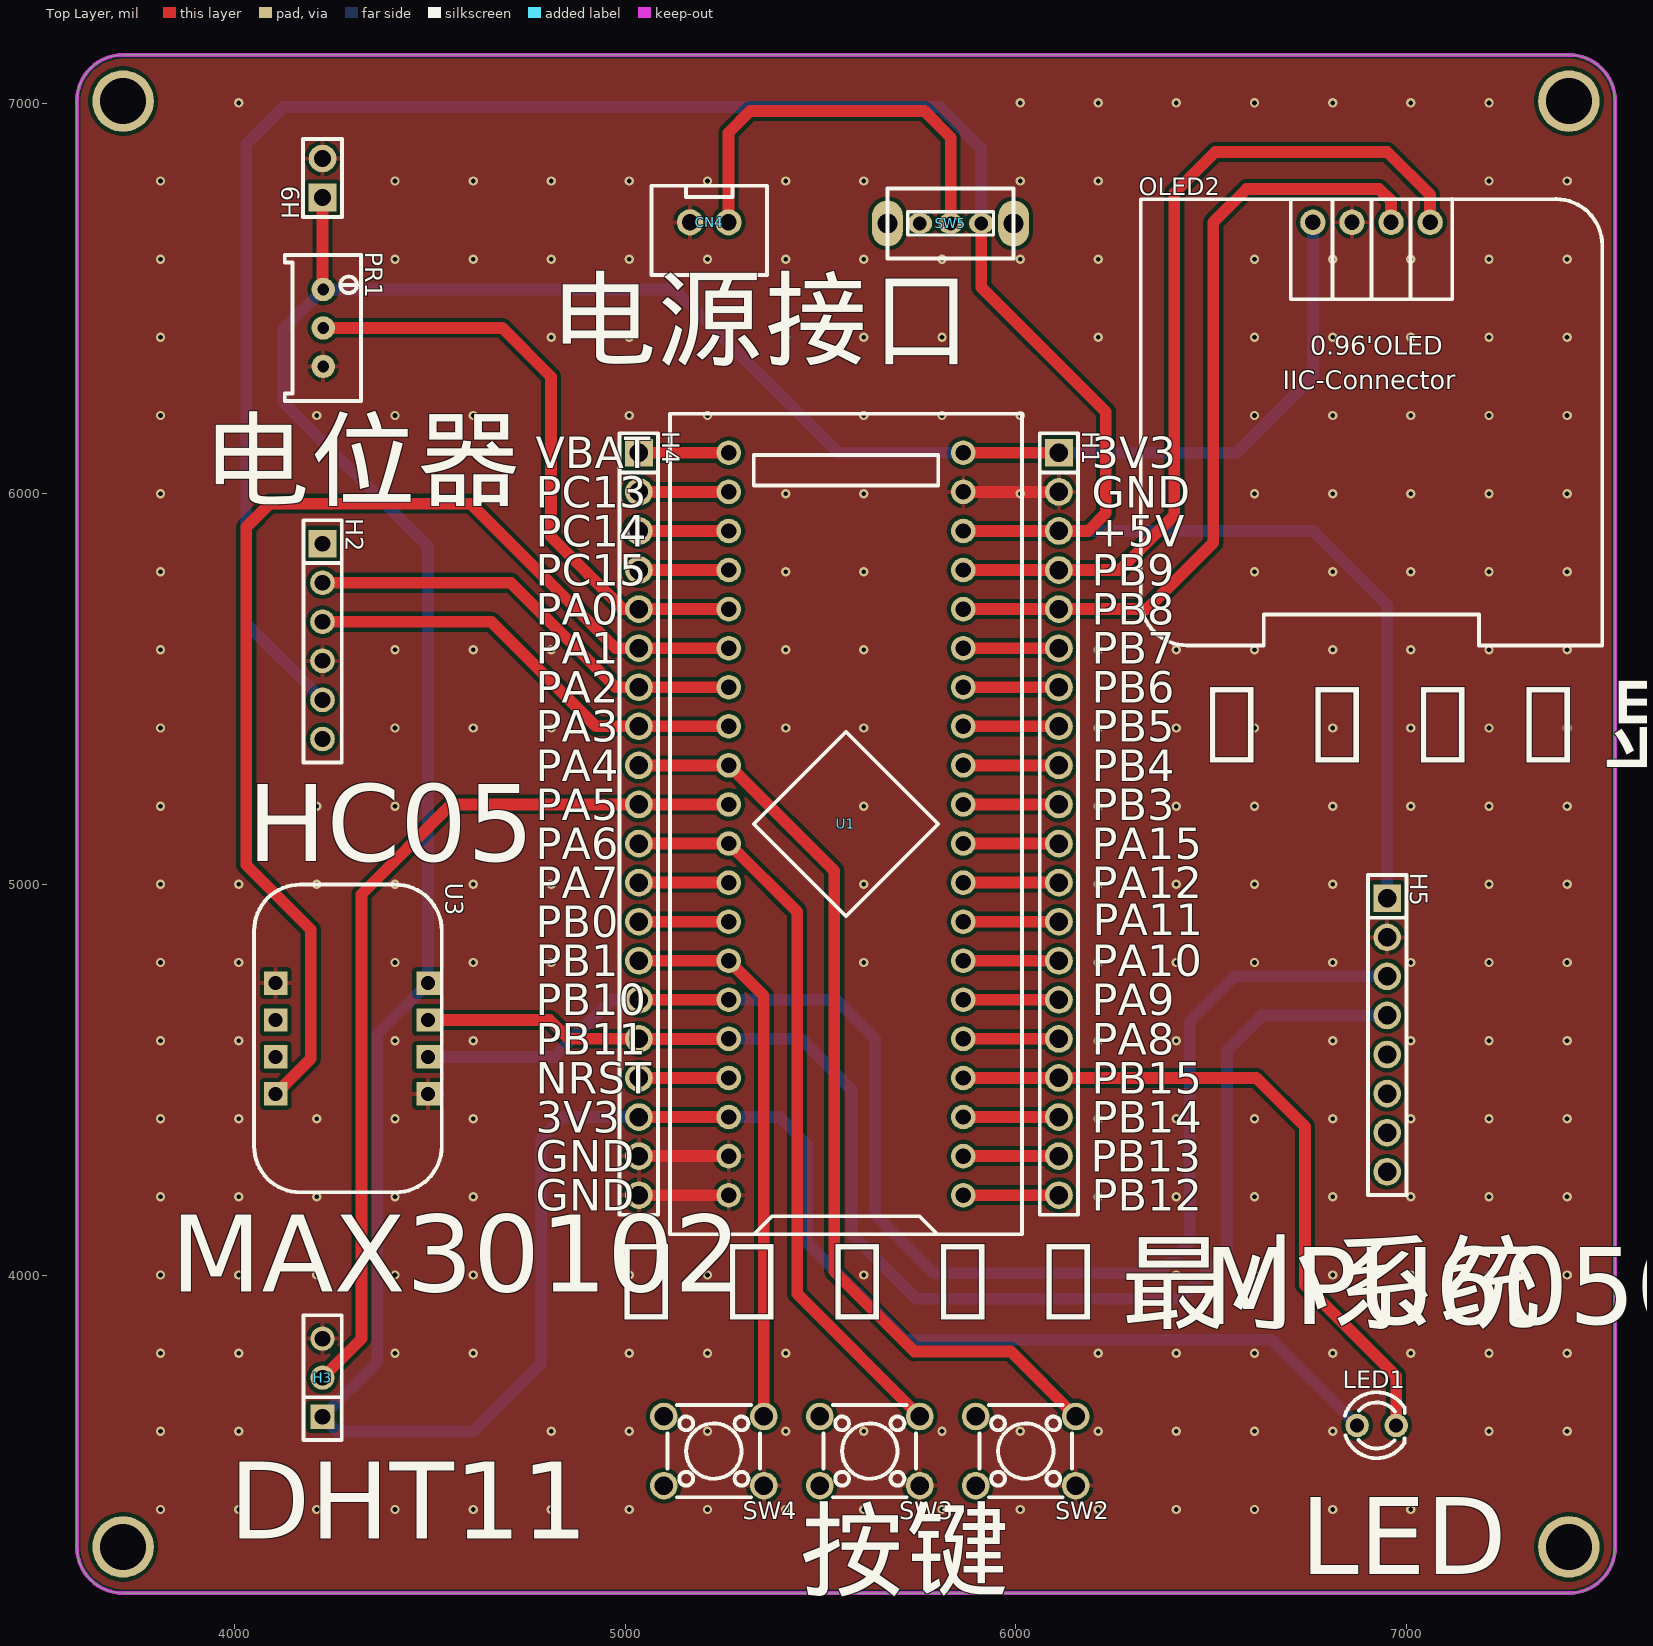
[diagram p0: Top Layer view]
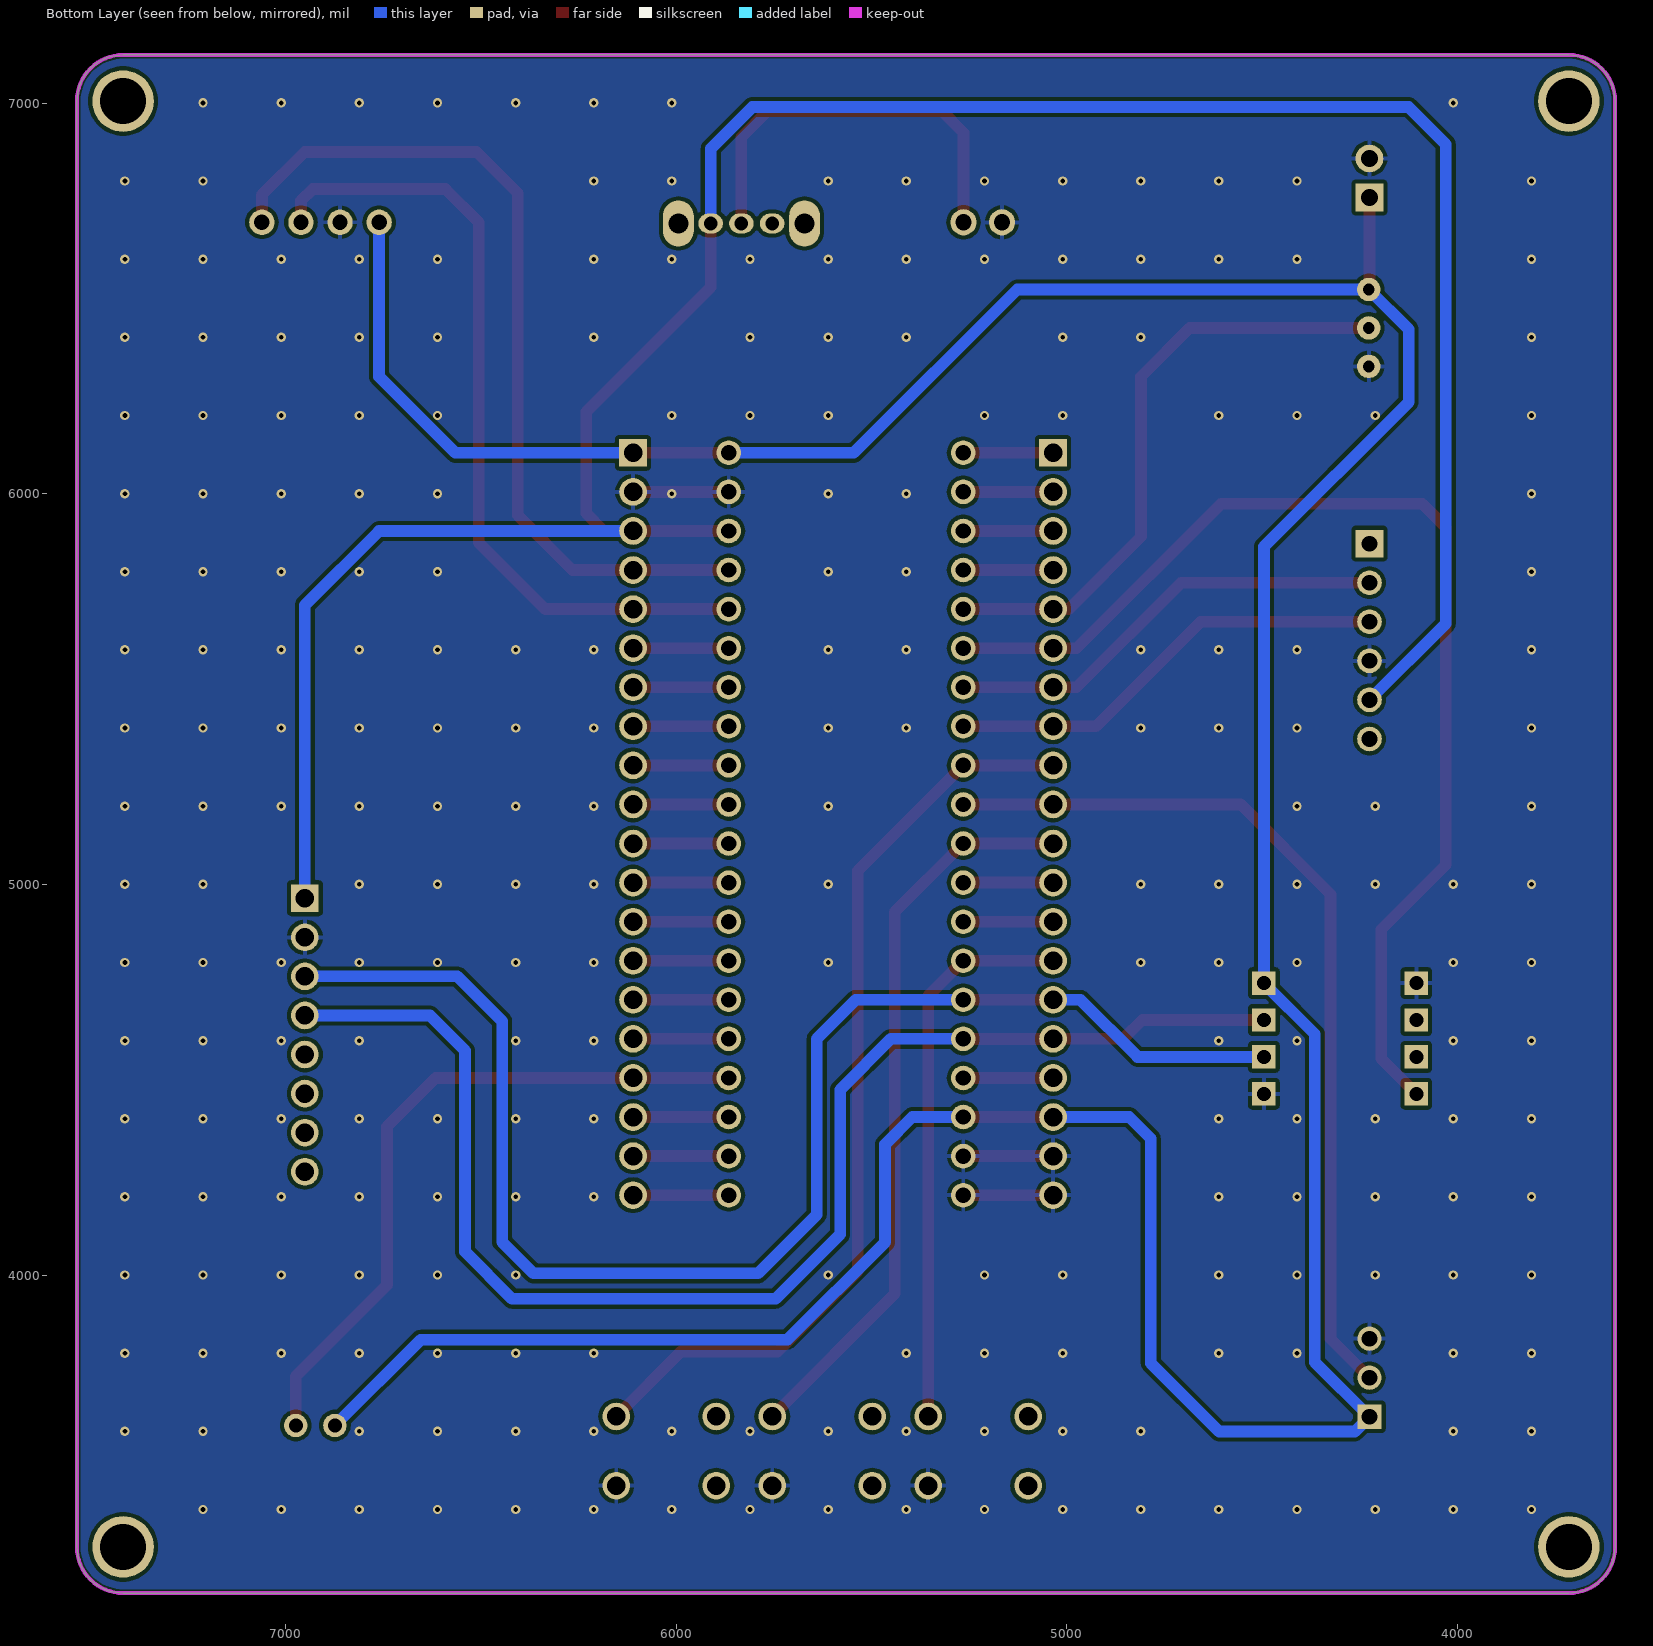
[diagram p1: Bottom Layer view, seen from below]
# Altium PCB MISC51261.pcbdoc
Units mil, origin at the board's own origin, x right, y up, seen from the top; angles counter-clockwise.
Board outline 3937.01 x 3937.01 mil, 2 copper layers (Top Layer, Bottom Layer), stack 62.206 mil thick; 16 components, 38 nets, 139 pads, 237 vias.

## Layer stack, top to bottom
Top Solder Mask Layer: solder mask 0.394, Dk 3.3
Top Layer: signal copper 1.379
Dielectric1: surface 59.449, FR4, Dk 4.5
Bottom Layer: signal copper 1.378
Bottom Solder Mask Layer: solder mask 0.394, Dk 3.3

## Board outline
3714.61,7123.5 ccw(c3714.61,7005.39) 3596.5,7005.39 3596.5,3304.61 ccw(c3714.61,3304.61) 3714.61,3186.5 7415.39,3186.5 ccw(c7415.39,3304.61) 7533.5,3304.61 7533.5,7005.39 ccw(c7415.39,7005.39) 7415.39,7123.5 3714.61,7123.5

## Design rules (kind name [scope] priority, off if disabled: settings)
BoardOutlineClearance copperThickness2oz_1 [All] p2 off: genericclearance=7.99 ignorepadtopadclearanceinfootprint=FALSE except(0: Arc-SplitContinuation Track-SplitContinuation SMDPad-SplitContinuation THPad-SplitContinuation Via-SplitContinuation Fill-SplitContinuation Region-SplitContinuation Poly-SplitContinuation Text-SplitContinuation Hole-SplitContinuation; 5.98: Arc-CutoutEdge Track-CutoutEdge SMDPad-CutoutEdge THPad-CutoutEdge Via-CutoutEdge Text-CutoutEdge; 6.9: Hole-OutlineEdge Hole-CutoutEdge; 10: Poly-OutlineEdge Poly-CutoutEdge; 11.81: Arc-OutlineEdge Track-OutlineEdge SMDPad-OutlineEdge THPad-OutlineEdge Via-OutlineEdge Fill-OutlineEdge Region-OutlineEdge Text-OutlineEdge Fill-CutoutEdge Region-CutoutEdge)
BoardOutlineClearance Plane_innerPlane_1 [All] p4 off: genericclearance=4.02 ignorepadtopadclearanceinfootprint=FALSE except(0: Arc-SplitContinuation Track-SplitContinuation SMDPad-SplitContinuation THPad-SplitContinuation Via-SplitContinuation Fill-SplitContinuation Region-SplitContinuation Poly-SplitContinuation Text-SplitContinuation Hole-SplitContinuation; 5.98: Arc-CutoutEdge Track-CutoutEdge SMDPad-CutoutEdge THPad-CutoutEdge Via-CutoutEdge Text-CutoutEdge; 6.9: Hole-OutlineEdge Hole-CutoutEdge; 10: Poly-OutlineEdge Poly-CutoutEdge; 11.81: Arc-OutlineEdge Track-OutlineEdge SMDPad-OutlineEdge THPad-OutlineEdge Via-OutlineEdge Fill-OutlineEdge Region-OutlineEdge Text-OutlineEdge Fill-CutoutEdge Region-CutoutEdge)
BoardOutlineClearance Copper_copperRegion_1 [All] p6 off: genericclearance=4.02 ignorepadtopadclearanceinfootprint=FALSE except(0: Arc-SplitContinuation Track-SplitContinuation SMDPad-SplitContinuation THPad-SplitContinuation Via-SplitContinuation Fill-SplitContinuation Region-SplitContinuation Poly-SplitContinuation Text-SplitContinuation Hole-SplitContinuation; 5.98: Arc-CutoutEdge Track-CutoutEdge SMDPad-CutoutEdge THPad-CutoutEdge Via-CutoutEdge Text-CutoutEdge; 6.9: Hole-OutlineEdge Hole-CutoutEdge; 10: Poly-OutlineEdge Poly-CutoutEdge; 11.81: Arc-OutlineEdge Track-OutlineEdge SMDPad-OutlineEdge THPad-OutlineEdge Via-OutlineEdge Fill-OutlineEdge Region-OutlineEdge Text-OutlineEdge Fill-CutoutEdge Region-CutoutEdge)
BoardOutlineClearance Copper_copperRegion_copperThickness1oz_1 [All] p8 off: genericclearance=4.02 ignorepadtopadclearanceinfootprint=FALSE except(0: Arc-SplitContinuation Track-SplitContinuation SMDPad-SplitContinuation THPad-SplitContinuation Via-SplitContinuation Fill-SplitContinuation Region-SplitContinuation Poly-SplitContinuation Text-SplitContinuation Hole-SplitContinuation; 5.98: Arc-CutoutEdge Track-CutoutEdge SMDPad-CutoutEdge THPad-CutoutEdge Via-CutoutEdge Text-CutoutEdge; 6.9: Hole-OutlineEdge Hole-CutoutEdge; 10: Poly-OutlineEdge Poly-CutoutEdge; 11.81: Arc-OutlineEdge Track-OutlineEdge SMDPad-OutlineEdge THPad-OutlineEdge Via-OutlineEdge Fill-OutlineEdge Region-OutlineEdge Text-OutlineEdge Fill-CutoutEdge Region-CutoutEdge)
BoardOutlineClearance Copper_copperRegion_Copper_copperRegion_1 [All] p10 off: genericclearance=4.02 ignorepadtopadclearanceinfootprint=FALSE except(0: Arc-SplitContinuation Track-SplitContinuation SMDPad-SplitContinuation THPad-SplitContinuation Via-SplitContinuation Fill-SplitContinuation Region-SplitContinuation Poly-SplitContinuation Text-SplitContinuation Hole-SplitContinuation; 5.98: Arc-CutoutEdge Track-CutoutEdge SMDPad-CutoutEdge THPad-CutoutEdge Via-CutoutEdge Text-CutoutEdge; 6.9: Hole-OutlineEdge Hole-CutoutEdge; 10: Poly-OutlineEdge Poly-CutoutEdge; 11.81: Arc-OutlineEdge Track-OutlineEdge SMDPad-OutlineEdge THPad-OutlineEdge Via-OutlineEdge Fill-OutlineEdge Region-OutlineEdge Text-OutlineEdge Fill-CutoutEdge Region-CutoutEdge)
BoardOutlineClearance copperThickness1oz_1 [All] p12: genericclearance=4.02 ignorepadtopadclearanceinfootprint=FALSE except(0: Arc-SplitContinuation Track-SplitContinuation SMDPad-SplitContinuation THPad-SplitContinuation Via-SplitContinuation Fill-SplitContinuation Region-SplitContinuation Poly-SplitContinuation Text-SplitContinuation Hole-SplitContinuation; 5.98: Arc-CutoutEdge Track-CutoutEdge SMDPad-CutoutEdge THPad-CutoutEdge Via-CutoutEdge Text-CutoutEdge; 6.9: Hole-OutlineEdge Hole-CutoutEdge; 10: Poly-OutlineEdge Poly-CutoutEdge; 11.81: Arc-OutlineEdge Track-OutlineEdge SMDPad-OutlineEdge THPad-OutlineEdge Via-OutlineEdge Fill-OutlineEdge Region-OutlineEdge Text-OutlineEdge Fill-CutoutEdge Region-CutoutEdge)
Clearance copperThickness2oz [All] p1 off: gap=7.99 ignorepadtopadclearanceinfootprint=FALSE except(5.98: SMDPad-Track SMDPad-SMDPad THPad-Track SMDPad-THPad THPad-THPad Track-Via SMDPad-Via THPad-Via Via-Via Fill-SMDPad Region-SMDPad Fill-THPad Region-THPad Fill-Via Region-Via Fill-Fill Fill-Region Region-Region Arc-Track Arc-SMDPad Arc-THPad Arc-Via Fill-Arc Region-Arc Arc-Arc Text-Track SMDPad-Text Text-THPad Text-Via Fill-Text Region-Text Arc-Text Text-Text; 6.9: Hole-Track Hole-SMDPad Hole-THPad Hole-Via Fill-Hole Region-Hole Hole-Arc Hole-Text; 10: Poly-Track Poly-SMDPad Poly-THPad Poly-Via Poly-Fill Poly-Region Poly-Poly Poly-Arc Poly-Text Poly-Hole; 11.81: Fill-Track Region-Track)
Clearance Plane_innerPlane [All] p3 off: gap=4.02 ignorepadtopadclearanceinfootprint=FALSE except(5.98: SMDPad-Track SMDPad-SMDPad THPad-Track SMDPad-THPad THPad-THPad Track-Via SMDPad-Via THPad-Via Via-Via Fill-SMDPad Region-SMDPad Fill-THPad Region-THPad Fill-Via Region-Via Fill-Fill Fill-Region Region-Region Arc-Track Arc-SMDPad Arc-THPad Arc-Via Fill-Arc Region-Arc Arc-Arc Text-Track SMDPad-Text Text-THPad Text-Via Fill-Text Region-Text Arc-Text Text-Text; 6.9: Hole-Track Hole-SMDPad Hole-THPad Hole-Via Fill-Hole Region-Hole Hole-Arc Hole-Text; 10: Poly-Track Poly-SMDPad Poly-THPad Poly-Via Poly-Fill Poly-Region Poly-Poly Poly-Arc Poly-Text Poly-Hole; 11.81: Fill-Track Region-Track)
Clearance Copper_copperRegion [All] p5 off: gap=4.02 ignorepadtopadclearanceinfootprint=FALSE except(5.98: SMDPad-Track SMDPad-SMDPad THPad-Track SMDPad-THPad THPad-THPad Track-Via SMDPad-Via THPad-Via Via-Via Fill-SMDPad Region-SMDPad Fill-THPad Region-THPad Fill-Via Region-Via Fill-Fill Fill-Region Region-Region Arc-Track Arc-SMDPad Arc-THPad Arc-Via Fill-Arc Region-Arc Arc-Arc Text-Track SMDPad-Text Text-THPad Text-Via Fill-Text Region-Text Arc-Text Text-Text; 6.9: Hole-Track Hole-SMDPad Hole-THPad Hole-Via Fill-Hole Region-Hole Hole-Arc Hole-Text; 10: Poly-Track Poly-SMDPad Poly-THPad Poly-Via Poly-Fill Poly-Region Poly-Poly Poly-Arc Poly-Text Poly-Hole; 11.81: Fill-Track Region-Track)
Clearance Copper_copperRegion_copperThickness1oz [All] p7 off: gap=4.02 ignorepadtopadclearanceinfootprint=FALSE except(5.98: SMDPad-Track SMDPad-SMDPad THPad-Track SMDPad-THPad THPad-THPad Track-Via SMDPad-Via THPad-Via Via-Via Fill-SMDPad Region-SMDPad Fill-THPad Region-THPad Fill-Via Region-Via Fill-Fill Fill-Region Region-Region Arc-Track Arc-SMDPad Arc-THPad Arc-Via Fill-Arc Region-Arc Arc-Arc Text-Track SMDPad-Text Text-THPad Text-Via Fill-Text Region-Text Arc-Text Text-Text; 6.9: Hole-Track Hole-SMDPad Hole-THPad Hole-Via Fill-Hole Region-Hole Hole-Arc Hole-Text; 10: Poly-Track Poly-SMDPad Poly-THPad Poly-Via Poly-Fill Poly-Region Poly-Poly Poly-Arc Poly-Text Poly-Hole; 11.81: Fill-Track Region-Track)
Clearance Copper_copperRegion_Copper_copperRegion [All] p9 off: gap=4.02 ignorepadtopadclearanceinfootprint=FALSE except(5.98: SMDPad-Track SMDPad-SMDPad THPad-Track SMDPad-THPad THPad-THPad Track-Via SMDPad-Via THPad-Via Via-Via Fill-SMDPad Region-SMDPad Fill-THPad Region-THPad Fill-Via Region-Via Fill-Fill Fill-Region Region-Region Arc-Track Arc-SMDPad Arc-THPad Arc-Via Fill-Arc Region-Arc Arc-Arc Text-Track SMDPad-Text Text-THPad Text-Via Fill-Text Region-Text Arc-Text Text-Text; 6.9: Hole-Track Hole-SMDPad Hole-THPad Hole-Via Fill-Hole Region-Hole Hole-Arc Hole-Text; 10: Poly-Track Poly-SMDPad Poly-THPad Poly-Via Poly-Fill Poly-Region Poly-Poly Poly-Arc Poly-Text Poly-Hole; 11.81: Fill-Track Region-Track)
Clearance copperThickness1oz [All] p11: gap=4.02 ignorepadtopadclearanceinfootprint=FALSE except(5.98: SMDPad-Track SMDPad-SMDPad THPad-Track SMDPad-THPad THPad-THPad Track-Via SMDPad-Via THPad-Via Via-Via Fill-SMDPad Region-SMDPad Fill-THPad Region-THPad Fill-Via Region-Via Fill-Fill Fill-Region Region-Region Arc-Track Arc-SMDPad Arc-THPad Arc-Via Fill-Arc Region-Arc Arc-Arc Text-Track SMDPad-Text Text-THPad Text-Via Fill-Text Region-Text Arc-Text Text-Text; 6.9: Hole-Track Hole-SMDPad Hole-THPad Hole-Via Fill-Hole Region-Hole Hole-Arc Hole-Text; 10: Poly-Track Poly-SMDPad Poly-THPad Poly-Via Poly-Fill Poly-Region Poly-Poly Poly-Arc Poly-Text Poly-Hole; 11.81: Fill-Track Region-Track)
DiffPairsRouting differentialPair [All] p1: maxlimit=6 minlimit=6 mostfreqgap=6 toplayer_minwidth=5 toplayer_prefwidth=10 toplayer_maxwidth=100 toplayer_mingap=6 toplayer_prefgap=6 toplayer_maxgap=6 bottomlayer_minwidth=5 bottomlayer_prefwidth=10 bottomlayer_maxwidth=100 bottomlayer_mingap=6 bottomlayer_prefgap=6 bottomlayer_maxgap=6 maxuncoupledlength=10
HoleToHoleClearance otherClearance [All] p1: gap=11.81 allowstackedmicrovias=TRUE
Length netLength [All] p1: minlimit=0 maxlimit=0
PasteMaskExpansion pasteMaskExpansion [All] p1: expansion=0
PlaneConnect innerPlane [All] p1: planeconnectstyle=Relief reliefexpansion=20 reliefentries=4 reliefconductorwidth=10 reliefairgap=10
PolygonConnect copperRegion_copperThickness1oz [All] p1 off: connectstyle=Relief reliefconductorwidth=10 reliefentries=4 polygonreliefangle="90 Angle" airgapwidth=10 via.connectstyle=Relief via.reliefconductorwidth=10 via.reliefentries=4 via.polygonreliefangle="90 Angle" via.airgapwidth=10
PolygonConnect copperRegion_Copper_copperRegion [All] p2 off: connectstyle=Relief reliefconductorwidth=10 reliefentries=4 polygonreliefangle="90 Angle" airgapwidth=10 via.connectstyle=Relief via.reliefconductorwidth=10 via.reliefentries=4 via.polygonreliefangle="90 Angle" via.airgapwidth=10
PolygonConnect copperRegion [All] p3: connectstyle=Relief reliefconductorwidth=10 reliefentries=4 polygonreliefangle="90 Angle" airgapwidth=10 via.connectstyle=Relief via.reliefconductorwidth=10 via.reliefentries=4 via.polygonreliefangle="90 Angle" via.airgapwidth=10
RoutingVias viaSize [All] p1: holewidth=12.01 width=24.02 viastyle="Through Hole" minholewidth=11.81 minwidth=19.68 maxholewidth=248.03 maxwidth=393.7
SolderMaskExpansion solderMaskExpansion [IsVia] p1: expansion=-1000 istentingtop=TRUE
SolderMaskExpansion solderMaskExpansion [All] p2: expansion=2 istentingtop=FALSE
Width copperThickness2oz_2 [All] p1 off: maxlimit=100 minlimit=8 preferedwidth=10
Width copperThickness1oz_2 [All] p2: maxlimit=100 minlimit=5 preferedwidth=10

## Components (designator, comment, footprint, x,y, rotation, side; value= is the part's Value field where it differs from the comment)
CN4 "XH2.54*2P_直插" CONN-TH_2P-P2.50-XH2.54-2P 5215,6695 r0 top
H1 "" HDR-TH_20P-P2.54-V-M-1 6110,5155 r270 top
H2 "" HDR-TH_6P-P2.54-V-F 4225.19,5622.55 r270 top
H3 "" HDR-TH_3P-P2.54-V-F 4225.19,3737.8 r90 top
H4 "" HDR-TH_20P-P2.54-V-M-1 5035,5155 r270 top
H5 "" HDR-TH_8P-P2.54-V-F-1 6950,4615 r270 top
H9 "" HDR-TH_2P-P2.54-V-M-1 4225.19,6808.3 r90 top
LED1 "" LED_TH-3mm 6923.13,3615.51 r0 top
OLED2 "" 0.96OLED_4P 6910,6695 r0 top
PR1 "10kΩ" R_3296 4231.89,6424.59 r270 top
SW2 "" SW-TH_4P-L6.0-W6.0-P4.50-LS6.5 6025,3550 r180 top
SW3 "" SW-TH_4P-L6.0-W6.0-P4.50-LS6.5 5625.86,3550 r180 top
SW4 "" SW-TH_4P-L6.0-W6.0-P4.50-LS6.5 5226.72,3550 r180 top
SW5 "" 拨动开关 5837.9,6692.05 r180 top
U1 "STM32F103C8T6-Card" CONN-TH_L53.3-W22.9_STM32F103C8T6-CARD 5565,5155 r90 top
U3 "MAX30102" MAX30102 4530.31,4999.77 r270 top

## Footprints (in the part's own frame and the unit in brackets; to place one, negate y for a bottom-side part, rotate by r counter-clockwise, add the part's x,y. Pads: shape width x height; smd on the part's side, far side on the other; paste and mask are expansions set on the pad)
0.96OLED_4P [mm]
  round 1.65 hole 1 copper offset 0,0: 1(-3.81,-0.001) 2(-1.27,0.002) 3(1.27,0.002) 4(3.81,0.002)
  silkscreen extent -15,-27.5 15,1.5
CONN-TH_2P-P2.50-XH2.54-2P [mm]
  round 1.7 hole 1.05 paste+0 mask+0.05: 1(1.25,0) 2(-1.25,0)
  silkscreen extent -3.75,-3.42 3.75,2.37
CONN-TH_L53.3-W22.9_STM32F103C8T6-CARD [mm]
  round 1.6 hole 1: 1(-24.13,-7.62) 2(-21.59,-7.62) 3(-19.05,-7.62) 4(-16.51,-7.62) 5(-13.97,-7.62) 6(-11.43,-7.62) 7(-8.89,-7.62) 8(-6.35,-7.62) 9(-3.81,-7.62) 10(-1.27,-7.62) 11(1.27,-7.62) 12(3.81,-7.62) 13(6.35,-7.62) 14(8.89,-7.62) 15(11.43,-7.62) 16(13.97,-7.62) 17(16.51,-7.62) 18(19.05,-7.62) 19(21.59,-7.62) 20(24.13,-7.62) 21(24.13,7.62) 22(21.59,7.62) 23(19.05,7.62) 24(16.51,7.62) 25(13.97,7.62) 26(11.43,7.62) 27(8.89,7.62) 28(6.35,7.62) 29(3.81,7.62) 30(1.27,7.62) 31(-1.27,7.62) 32(-3.81,7.62) 33(-6.35,7.62) 34(-8.89,7.62) 35(-11.43,7.62) 36(-13.97,7.62) 37(-16.51,7.62) 38(-19.05,7.62) 39(-21.59,7.62) 40(-24.13,7.62)
  silkscreen extent -26.67,-11.43 26.67,11.43
HDR-TH_2P-P2.54-V-M-1 [mm]
  rect 1.8x1.8 hole 1.1: 1(-1.27,0)
  round 1.8 hole 1.1: 2(1.27,0)
  silkscreen extent -2.54,-1.27 2.54,1.27
HDR-TH_3P-P2.54-V-F [mil]
  rect 62x62 hole 40.16: 1(-100,0)
  round 62 hole 40.16: 2(0,0) 3(100,0)
  silkscreen extent -160,-49 160,49
HDR-TH_6P-P2.54-V-F [mm]
  rect 1.8x1.8 hole 1.02: 1(-6.35,0)
  round 1.6 hole 1.02: 2(-3.81,0) 3(-1.27,0) 4(1.27,0) 5(3.81,0) 6(6.35,0)
  silkscreen extent -7.87,-1.25 7.87,1.25
HDR-TH_8P-P2.54-V-F-1 [mm]
  rect 1.8x1.8 hole 1.2: 1(-8.89,0)
  round 1.8 hole 1.2: 2(-6.35,0) 3(-3.81,0) 4(-1.27,0) 5(1.27,0) 6(3.81,0) 7(6.35,0) 8(8.89,0)
  silkscreen extent -10.41,-1.25 10.41,1.25
HDR-TH_20P-P2.54-V-M-1 [mm]
  rect 1.8x1.8 hole 1.2: 1(-24.13,0)
  round 1.8 hole 1.2: 2(-21.59,0) 3(-19.05,0) 4(-16.51,0) 5(-13.97,0) 6(-11.43,0) 7(-8.89,0) 8(-6.35,0) 9(-3.81,0) 10(-1.27,0) 11(1.27,0) 12(3.81,0) 13(6.35,0) 14(8.89,0) 15(11.43,0) 16(13.97,0) 17(16.51,0) 18(19.05,0) 19(21.59,0) 20(24.13,0)
  silkscreen extent -25.4,-1.25 25.4,1.25
LED_TH-3mm [mil]
  round 60 hole 36 paste+0 mask+2: 1(-50,0) 2(50,0)
  silkscreen extent -81,-84 72,85
MAX30102 [mil]
  rect 60x60 hole 36: 1(251.97,-35) 2(346.46,-35) 3(440.94,-35) 4(535.43,-35) 5(251.97,-425) 6(346.46,-425) 7(440.94,-425) 8(535.43,-425)
  silkscreen extent 0,-480 787,0
R_3296 [mil]
  round 60 hole 30 paste+0 mask+2: 1(-98.4,-5) 2(0,-5) 3(98.4,-5)
  silkscreen extent -187,-103 187,92
SW-TH_4P-L6.0-W6.0-P4.50-LS6.5 [mm]
  round 1.8 hole 1.2: 1(-3.25,2.25) 2(3.25,2.25) 3(-3.25,-2.25) 4(3.25,-2.25)
  silkscreen extent -3,-3 3,3
拨动开关 [mil]
  oval 63x51.2 hole 35.4 paste+0 mask+2: 1(-73.4,0) 2(5,0) 3(84,0)
  oval 78.7x118.1 hole 51.2 paste+0 mask+2: 4(166.7,0) 5(-156.1,0)
  silkscreen extent -156,-90 167,90

## Free pads (board coordinates)
  round 157.48 hole 118.11: 1(3714.61,7005.39) 1(3714.61,3304.61) 1(7415.39,7005.39) 1(7415.39,3304.61)

## Via types
v1: diameter 24.02, hole 12, Top Layer to Bottom Layer, 237 vias

## Nets (pads, with @x,y where several pads share a name; then routed paths per layer and width w, separated by ;. In a path a pad name is that pad's centre, name@x,y a point inside that pad or via, vN(x,y) a via of type N, cw(c..) or ccw(c..) an arc to the next point about the centre after c; other vN are vias at no path point)
$1N17118: CN4.1 SW5.2 | length 1069.2
  Top Layer w30: CN4.1 5264.22,6924.22 5320,6980 5765,6980 5832.9,6912.1 SW5.2
+5V: H1.3 H2.5 H5.1 SW5.1 U1.18 | length 6586
  Top Layer w30: U1.18 H1.3 6185,5905 6230,5950 6230,6210 5911.3,6528.7 SW5.1
  Bottom Layer w30: H2.5 4030,5667.75 4030,6895 4125,6990 5805,6990 5911.3,6883.7 SW5.1 ; H1.3 6760,5905 6950,5715 H5.1
GND: CN4.2 H1.2 H2.4 H3.3 H4.19 H4.20 H5.2 H9.2 OLED2.2 PR1.3 SW2.1 SW3.1 SW4.1 U1.19 U1.39 U1.40 U3.4 U3.5 | length 715
  Top Layer w30: H4.20 U1.40@5270,4205 ; H4.19 U1.39@5270,4305 ; U1.19 H1.2
  other v1: 3810.6,3400.6 4010.6,3400.6 4210.6,3400.6 4410.6,3400.6 4610.6,3400.6 4810.6,3400.6 5010.6,3400.6 5210.6,3400.6 5410.6,3400.6 5610.6,3400.6 5810.6,3400.6 6010.6,3400.6 6210.6,3400.6 6410.6,3400.6 6610.6,3400.6 6810.6,3400.6 7010.6,3400.6 7210.6,3400.6 3810.6,3600.6 4010.6,3600.6 4810.6,3600.6 5010.6,3600.6 5210.6,3600.6 5410.6,3600.6 5610.6,3600.6 5810.6,3600.6 6010.6,3600.6 6210.6,3600.6 6410.6,3600.6 6610.6,3600.6 6810.6,3600.6 7210.6,3600.6 7410.6,3600.6 3810.6,3800.6 4010.6,3800.6 4410.6,3800.6 4610.6,3800.6 5010.6,3800.6 5210.6,3800.6 5410.6,3800.6 6210.6,3800.6 6410.6,3800.6 6610.6,3800.6 6810.6,3800.6 7010.6,3800.6 7210.6,3800.6 7410.6,3800.6 3810.6,4000.6 4010.6,4000.6 4210.6,4000.6 4410.6,4000.6 4610.6,4000.6 5010.6,4000.6 5210.6,4000.6 5610.6,4000.6 6410.6,4000.6 6610.6,4000.6 6810.6,4000.6 7010.6,4000.6 7210.6,4000.6 7410.6,4000.6 3810.6,4200.6 4010.6,4200.6 4210.6,4200.6 4410.6,4200.6 4610.6,4200.6 6210.6,4200.6 6410.6,4200.6 6610.6,4200.6 6810.6,4200.6 7010.6,4200.6 7210.6,4200.6 7410.6,4200.6 3810.6,4400.6 4010.6,4400.6 4210.6,4400.6 4410.6,4400.6 4610.6,4400.6 6210.6,4400.6 6410.6,4400.6 6610.6,4400.6 6810.6,4400.6 7010.6,4400.6 7210.6,4400.6 7410.6,4400.6 3810.6,4600.6 4010.6,4600.6 4410.6,4600.6 4610.6,4600.6 6210.6,4600.6 6410.6,4600.6 6810.6,4600.6 7010.6,4600.6 7210.6,4600.6 7410.6,4600.6 3810.6,4800.6 4010.6,4800.6 4410.6,4800.6 4610.6,4800.6 4810.6,4800.6 5610.6,4800.6 6210.6,4800.6 6410.6,4800.6 6610.6,4800.6 6810.6,4800.6 7010.6,4800.6 7210.6,4800.6 7410.6,4800.6 3810.6,5000.6 4010.6,5000.6 4210.6,5000.6 4410.6,5000.6 4610.6,5000.6 4810.6,5000.6 5610.6,5000.6 6210.6,5000.6 6410.6,5000.6 6610.6,5000.6 6810.6,5000.6 7210.6,5000.6 7410.6,5000.6 3810.6,5200.6 4210.6,5200.6 4410.6,5200.6 5610.6,5200.6 6210.6,5200.6 6410.6,5200.6 6610.6,5200.6 6810.6,5200.6 7010.6,5200.6 7210.6,5200.6 7410.6,5200.6 3810.6,5400.6 4410.6,5400.6 4610.6,5400.6 4810.6,5400.6 5410.6,5400.6 5610.6,5400.6 6210.6,5400.6 6410.6,5400.6 6610.6,5400.6 6810.6,5400.6 7010.6,5400.6 7210.6,5400.6 7410.6,5400.6 3810.6,5600.6 4410.6,5600.6 4610.6,5600.6 4810.6,5600.6 5410.6,5600.6 5610.6,5600.6 6210.6,5600.6 6410.6,5600.6 6610.6,5600.6 6810.6,5600.6 7010.6,5600.6 7210.6,5600.6 7410.6,5600.6 3810.6,5800.6 5410.6,5800.6 5610.6,5800.6 6610.6,5800.6 6810.6,5800.6 7010.6,5800.6 7210.6,5800.6 7410.6,5800.6 3810.6,6000.6 5410.6,6000.6 5610.6,6000.6 6010.6,6000.6 6610.6,6000.6 6810.6,6000.6 7010.6,6000.6 7210.6,6000.6 7410.6,6000.6 3810.6,6200.6 4210.6,6200.6 4410.6,6200.6 4610.6,6200.6 5010.6,6200.6 5210.6,6200.6 5610.6,6200.6 5810.6,6200.6 6010.6,6200.6 6610.6,6200.6 6810.6,6200.6 7010.6,6200.6 7210.6,6200.6 7410.6,6200.6 3810.6,6400.6 4810.6,6400.6 5010.6,6400.6 5410.6,6400.6 5610.6,6400.6 5810.6,6400.6 6210.6,6400.6 6610.6,6400.6 6810.6,6400.6 7010.6,6400.6 7210.6,6400.6 7410.6,6400.6 3810.6,6600.6 4410.6,6600.6 4610.6,6600.6 4810.6,6600.6 5010.6,6600.6 5210.6,6600.6 5410.6,6600.6 5610.6,6600.6 5810.6,6600.6 6010.6,6600.6 6210.6,6600.6 6610.6,6600.6 6810.6,6600.6 7010.6,6600.6 7210.6,6600.6 7410.6,6600.6 3810.6,6800.6 4410.6,6800.6 4610.6,6800.6 4810.6,6800.6 5010.6,6800.6 5210.6,6800.6 5410.6,6800.6 5610.6,6800.6 6010.6,6800.6 6210.6,6800.6 7210.6,6800.6 7410.6,6800.6 4010.6,7000.6 6010.6,7000.6 6210.6,7000.6 6410.6,7000.6 6610.6,7000.6 6810.6,7000.6 7010.6,7000.6 7210.6,7000.6
NRST: H4.17 U1.37 | length 235
  Top Layer w30: H4.17 U1.37@5270,4505
PA0: H4.5 PR1.2 U1.25 | length 1581.3
  Top Layer w30: PR1.2 4685.41,6424.59 4810,6300 4810,5890 4995,5705 H4.5 U1.25@5270,5705
PA1: H4.6 U1.26 U3.8 | length 2974.3
  Top Layer w30: U3.8 4195,4554.03 4195,4885 4030,5050 4030,5915 4090,5975 4605,5975 4975,5605 H4.6 U1.26@5270,5605
PA2: H2.2 H4.7 U1.27 | length 1155.6
  Top Layer w30: H2.2 4707.45,5772.55 4975,5505 H4.7 U1.27@5270,5505
PA3: H2.3 H4.8 U1.28 | length 1155.6
  Top Layer w30: H2.3 4657.45,5672.55 4925,5405 H4.8 U1.28@5270,5405
PA4: H4.9 SW2.3 U1.29 | length 2410.1
  Top Layer w30: H4.9 U1.29 U1.29@5270,5305 ; U1.29@5267.5,5302.5 5535,5035 5535,4010 5740,3805 5986.53,3805 SW2.3
PA5: H3.2 H4.10 U1.30 | length 2318.8
  Top Layer w30: H3.2 4325,3837.61 4325,4975 4555,5205 H4.10 U1.30@5270,5205
PA6: H4.11 SW3.3 U1.31 | length 1900.4
  Top Layer w30: H4.11 U1.31 U1.31@5270,5105 ; U1.31@5267.5,5102.5 5440,4930 5440,3952.39 SW3.3
PA7: H4.12 U1.32 | length 235
  Top Layer w30: H4.12 U1.32@5270,5005
PA8: H1.16 U1.5 | length 245
  Top Layer w30: U1.5 H1.16
PA9: H1.15 U1.6 | length 245
  Top Layer w30: U1.6 H1.15
PA10: H1.14 U1.7 | length 245
  Top Layer w30: U1.7 H1.14
PA11: H1.13 U1.8 | length 245
  Top Layer w30: U1.8 H1.13
PA12: H1.12 U1.9 | length 245
  Top Layer w30: U1.9 H1.12
PA15: H1.11 U1.10 | length 245
  Top Layer w30: U1.10 H1.11
PB0: H4.13 U1.33 | length 235
  Top Layer w30: H4.13 U1.33@5270,4905
PB1: H4.14 SW4.3 U1.34 | length 1435
  Top Layer w30: H4.14 U1.34 U1.34@5270,4805 ; U1.34@5267.5,4802.5 5354.67,4715.33 SW4.3
PB3: H1.10 U1.11 | length 245
  Top Layer w30: U1.11 H1.10
PB4: H1.9 U1.12 | length 245
  Top Layer w30: U1.12 H1.9
PB5: H1.8 U1.13 | length 245
  Top Layer w30: U1.13 H1.8
PB6: H1.7 U1.14 | length 245
  Top Layer w30: U1.14 H1.7
PB7: H1.6 U1.15 | length 245
  Top Layer w30: U1.15 H1.6
PB8: H1.5 OLED2.3 U1.16 | length 2088
  Top Layer w30: U1.16 H1.5 6335,5705 6505,5875 6505,6695 6590,6780 6930,6780 6960,6750 OLED2.3@6960,6695.05
PB9: H1.4 OLED2.4 U1.17 | length 2237
  Top Layer w30: U1.17 H1.4 6265,5805 6405,5945 6405,6770 6510,6875 6950,6875 7060,6765 OLED2.4@7060,6695.05
PB10: H4.15 H5.3 U1.35 U3.3 | length 3719.6
  Top Layer w30: H4.15 U1.35@5270,4705
  Bottom Layer w30: U3.3 4818.83,4558.83 4965,4705 H4.15 ; U1.35 5540,4705 5640,4605 5640,4155 5790,4005 6365,4005 6445,4085 6445,4650 6560,4765 H5.3
PB11: H4.16 H5.4 U1.36 U3.2 | length 3573.9
  Top Layer w30: U3.2 4806.69,4653.31 4855,4605 H4.16 U1.36@5270,4605
  Bottom Layer w30: U1.36 5450,4605 5580,4475 5580,4105 5745,3940 6420,3940 6540,4060 6540,4575 6630,4665 H5.4
PB12: H1.20 U1.1 | length 245
  Top Layer w30: U1.1 H1.20
PB13: H1.19 U1.2 | length 245
  Top Layer w30: U1.2 H1.19
PB14: H1.18 U1.3 | length 245
  Top Layer w30: U1.3 H1.18
PB15: H1.17 LED1.2 U1.4 | length 1787.8
  Top Layer w30: U1.4 H1.17 6615,4505 6740,4380 6740,3975 6973.13,3741.87 LED1.2
PC13: H4.2 U1.22 | length 235
  Top Layer w30: H4.2 U1.22@5270,6005
PC14: H4.3 U1.23 | length 235
  Top Layer w30: H4.3 U1.23@5270,5905
PC15: H4.4 U1.24 | length 235
  Top Layer w30: H4.4 U1.24@5270,5805
VBAT: H4.1 U1.21 | length 235
  Top Layer w30: H4.1 U1.21@5270,6105
VCC: H1.1 H3.1 H4.18 H9.1 LED1.1 OLED2.1 PR1.1 U1.20 U1.38 U3.1 | length 10423
  Top Layer w30: H9.1 4225.19,6524.69 PR1.1 ; H4.18 U1.38@5270,4405 ; U1.20 H1.1
  Bottom Layer w30: H4.18 4840,4405 4785,4350 4785,3775 4610,3600 4262.99,3600 H3.1 4365,3777.61 4365,4617.49 U3.1 4495.31,5864.69 4125,6235 4125,6421.09 PR1.1 5127.01,6522.99 5545,6105 U1.20 ; U1.38 5395,4405 5465,4335 5465,4085 5715,3835 6653.64,3835 LED1.1 ; H1.1 6565,6105 6760,6300 OLED2.1
pads on no net: H2.1 H2.6 H5.5 H5.6 H5.7 H5.8 SW2.2 SW2.4 SW3.2 SW3.4 SW4.2 SW4.4 SW5.3 SW5.4 SW5.5 U3.6 U3.7

## Polygon pours and split planes (outlines as drawn)
GND on Bottom Layer (solid, remove dead copper, pour order 2): 3525,7245 3525,3080 7700,3080 7700,7245
GND on Top Layer (solid, remove dead copper, pour order 2): 3000,7415 3000,3000 7930,3000 7930,7415

## Keep-outs
Board Outline Layer:
  the board outline again, w10

## Silkscreen, mask and mechanical layers (free items; w line width, h text height)
Top Silkscreen Layer:
  text "电源接口" at 4812.87,6351.57 h196.85
  text "VBAT" at 4770.95,6065 h80
  text "3V3" at 6194.16,6065 h80
  text "电位器" at 3925.14,5992.98 h196.85
  text "PC13" at 4770.95,5965 h80
  text "GND" at 6194.16,5965 h80
  text "PC14" at 4770.95,5865 h80
  text "+5V" at 6194.16,5865 h80
  text "PC15" at 4770.95,5765 h80
  text "PB9" at 6194.16,5765 h80
  text "PA0" at 4770.95,5665 h80
  text "PB8" at 6194.16,5665 h80
  text "PA1" at 4770.95,5565 h80
  text "PB7" at 6194.16,5565 h80
  text "PA2" at 4770.95,5465 h80
  text "PB6" at 6194.16,5465 h80
  text "PA3" at 4770.95,5365 h80
  text "PB5" at 6194.16,5365 h80
  text "Oled显示器" at 6418.02,5311.19 h196.85
  text "PA4" at 4770.95,5265 h80
  text "PB4" at 6194.16,5265 h80
  text "PA5" at 4770.95,5165 h80
  text "PB3" at 6194.16,5165 h80
  text "PA6" at 4770.95,5065 h80
  text "PA15" at 6194.16,5065 h80
  text "HC05" at 4033.11,5059.75 h196.85
  text "PA7" at 4770.95,4965 h80
  text "PA12" at 6194.16,4965 h80
  text "PA11" at 6195.95,4870 h80
  text "PB0" at 4770.95,4865 h80
  text "PB1" at 4770.95,4765 h80
  text "PA10" at 6194.16,4765 h80
  text "PB10" at 4770.95,4665 h80
  text "PA9" at 6194.16,4665 h80
  text "PB11" at 4770.95,4565 h80
  text "PA8" at 6194.16,4565 h80
  text "NRST" at 4770.95,4465 h80
  text "PB15" at 6194.16,4465 h80
  text "3V3" at 4770.95,4365 h80
  text "PB14" at 6194.16,4365 h80
  text "GND" at 4770.95,4265 h80
  text "PB13" at 6190.95,4265 h80
  text "GND" at 4770.95,4165 h80
  text "PB12" at 6194.16,4165 h80
  text "MAX30102" at 3837.01,3957.62 h196.85
  text "STM32最小系统" at 4919.45,3886.57 h196.85
  text "MPU6050" at 6480,3875 h196.85
  text "DHT11" at 3986.59,3325 h196.85
  text "LED" at 6727.92,3235 h196.85
  text "按键" at 5446.3,3203.15 h196.85